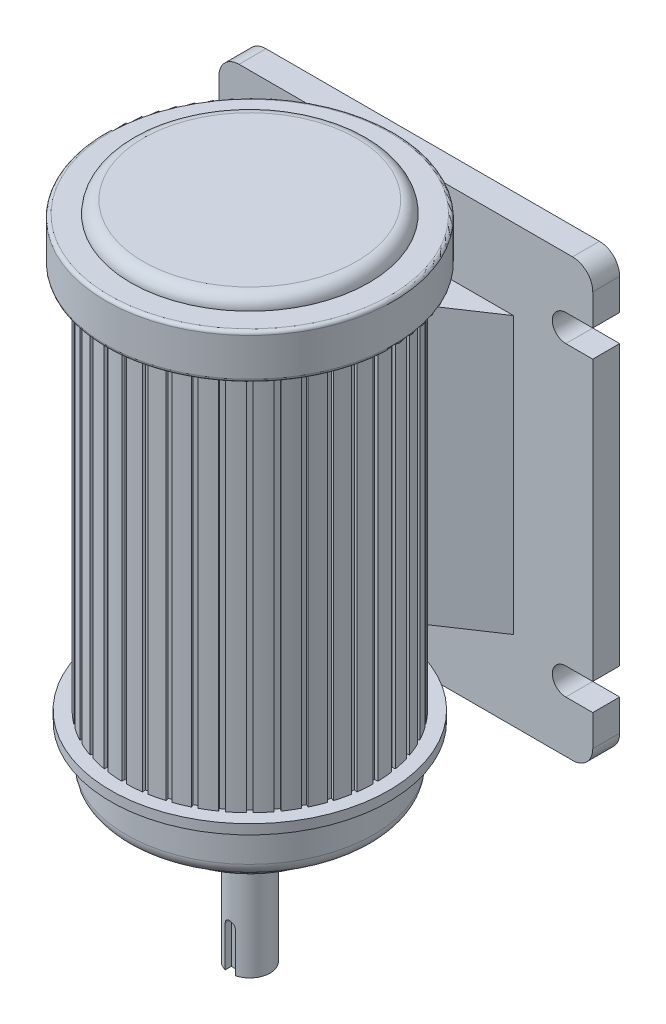
from build123d import *

# Parameters (mm, degrees)
SKETCH1_W           = 55.500789996
SKETCH1_H           = 64.737092018
BOSS_EXTRUDE1_DEPTH = 4
CUT_EXTRUDE1_DEPTH  = 4
FILLET1_R           = 3
CUT_EXTRUDE2_DEPTH  = 57.141911971
BOSS_EXTRUDE2_DEPTH = 20.5
SKETCH7_R           = 4.533623048
SKETCH7_R_2         = 3.951109074
BOSS_EXTRUDE3_DEPTH = 0.5
SKETCH8_R           = 3
BOSS_EXTRUDE4_DEPTH = 20
SKETCH9_W           = 1.5
SKETCH9_H           = 2
CUT_EXTRUDE3_DEPTH  = 6
SKETCH10_R          = 0.75
CUT_EXTRUDE4_DEPTH  = 2


with BuildPart() as part:
    # Sketch1 → Boss-Extrude1 (new body)
    with BuildSketch(Plane.XY):
        with Locations((9.22608239, 110.038628539)):
            Rectangle(SKETCH1_W, SKETCH1_H)
    extrude(amount=BOSS_EXTRUDE1_DEPTH)

    # Sketch2 → Cut-Extrude1 (cut)
    with BuildSketch(Plane.XY.offset(4)):
        with BuildLine():
            Line((-14.527141875, 134.7549071), (-18.524312608, 134.7549071))
            Line((-18.524312608, 134.7549071), (-18.524312608, 130.7549071))
            Line((-18.524312608, 130.7549071), (-14.527141875, 130.7549071))
            ThreePointArc((-14.527141875, 130.7549071), (-12.527141875, 132.7549071), (-14.527141875, 134.7549071))
        make_face()
        with BuildLine():
            Line((-18.524312608, 89.322349977), (-18.524312608, 85.322349977))
            Line((-18.524312608, 85.322349977), (-14.527141875, 85.322349977))
            ThreePointArc((-14.527141875, 85.322349977), (-12.527141875, 87.322349977), (-14.527141875, 89.322349977))
            Line((-14.527141875, 89.322349977), (-18.524312608, 89.322349977))
        make_face()
        with BuildLine():
            Line((36.976477388, 130.7549071), (36.976477388, 134.7549071))
            Line((36.976477388, 134.7549071), (32.979306656, 134.7549071))
            ThreePointArc((32.979306656, 134.7549071), (30.979306656, 132.7549071), (32.979306656, 130.7549071))
            Line((32.979306656, 130.7549071), (36.976477388, 130.7549071))
        make_face()
        with BuildLine():
            Line((36.976477388, 85.322349977), (36.976477388, 89.322349977))
            Line((36.976477388, 89.322349977), (32.979306656, 89.322349977))
            ThreePointArc((32.979306656, 89.322349977), (30.979306656, 87.322349977), (32.979306656, 85.322349977))
            Line((32.979306656, 85.322349977), (36.976477388, 85.322349977))
        make_face()
    extrude(amount=-CUT_EXTRUDE1_DEPTH, mode=Mode.SUBTRACT)

    # Fillet1
    fillet1_edges = [part.edges().sort_by_distance(p)[0] for p in [
        (36.976477388, 77.67008253, 2),
        (-18.524312608, 77.67008253, 2),
        (-18.524312608, 142.407174548, 2),
        (36.976477388, 142.407174548, 2),
    ]]
    fillet(fillet1_edges, radius=FILLET1_R)



with BuildPart() as body_2:
    # Sketch3 → Revolve1 (revolve)
    with BuildSketch(Plane(origin=(9.22608239, -4.248250363, 39.612036091), x_dir=(0, 1, 0), z_dir=(1, 0, 0)), mode=Mode.PRIVATE) as revolve1_sk:
        with BuildLine():
            Line((75.270637963, -12.45948374), (153.17887773, -12.45948374))
            Line((153.17887773, -12.45948374), (153.17887773, 3.386494149))
            ThreePointArc((153.17887773, 3.386494149), (152.644055983, 4.677668063), (151.352882069, 5.21248981))
            Line((151.352882069, 5.21248981), (151.352882069, 8.408578473))
            ThreePointArc((151.352882069, 8.408578473), (151.206435459, 8.762131864), (150.852882069, 8.908578473))
            Line((150.852882069, 8.908578473), (145.22638088, 8.908578473))
            ThreePointArc((145.22638088, 8.908578473), (144.872827489, 8.762131864), (144.72638088, 8.408578473))
            Line((144.72638088, 8.408578473), (144.72638088, 6.1906691))
            Line((144.72638088, 6.1906691), (87.584468909, 6.1906691))
            Line((87.584468909, 6.1906691), (87.584468909, 8.192651448))
            Line((87.584468909, 8.192651448), (86.141891274, 8.192651448))
            Line((86.141891274, 8.192651448), (86.141891274, 7.166046123))
            Line((86.141891274, 7.166046123), (86.141891274, 5.883061514))
            Line((86.141891274, 5.883061514), (80.722831843, 5.883061514))
            ThreePointArc((80.722831843, 5.883061514), (79.308618281, 5.297275076), (78.722831843, 3.883061514))
            Line((78.722831843, 3.883061514), (78.722831843, -0.040180747))
            Line((78.722831843, -0.040180747), (77.843708387, -0.682232562))
            Line((77.843708387, -0.682232562), (77.843708387, 0.737127384))
            ThreePointArc((77.843708387, 0.737127384), (77.785129743, 0.878548741), (77.643708387, 0.937127384))
            Line((77.643708387, 0.937127384), (76.752066951, 0.937127384))
            ThreePointArc((76.752066951, 0.937127384), (76.610645595, 0.878548741), (76.552066951, 0.737127384))
            Line((76.552066951, 0.737127384), (76.552066951, 0.029558387))
            Line((76.552066951, 0.029558387), (75.470637963, 0.029558387))
            ThreePointArc((75.470637963, 0.029558387), (75.329216607, -0.029020257), (75.270637963, -0.170441613))
            Line((75.270637963, -0.170441613), (75.270637963, -12.45948374))
        make_face()
    revolve(revolve1_sk.sketch.rotate(Axis((9.22608239, 71.0223876, 27.152552351), (0, 1, 0)), 180), axis=Axis((9.22608239, 71.0223876, 27.152552351), (0, 1, 0)))

    # Sketch5 → Cut-Extrude2 (cut)
    with BuildSketch(Plane(origin=(0, 83.336218546, 0), x_dir=(1, 0, 0), z_dir=(0, 1, 0))):
        with BuildLine():
            Line((11.788472717, -8.679264697), (11.714933059, -9.143575829))
            Line((11.714933059, -9.143575829), (12.424124541, -9.255900725))
            Line((12.424124541, -9.255900725), (12.4976642, -8.791589593))
            ThreePointArc((12.4976642, -8.791589593), (12.143609073, -8.732013841), (11.788472717, -8.679264697))
        make_face()
        with BuildLine():
            Line((8.867066569, -8.505855363), (8.867066569, -8.975954192))
            Line((8.867066569, -8.975954192), (9.585098212, -8.975954192))
            Line((9.585098212, -8.975954192), (9.585098212, -8.505855363))
            ThreePointArc((9.585098212, -8.505855363), (9.22608239, -8.502399512), (8.867066569, -8.505855363))
        make_face()
        with BuildLine():
            Line((14.646784312, -9.307547683), (14.501515785, -9.754638237))
            Line((14.501515785, -9.754638237), (15.184404458, -9.976522218))
            Line((15.184404458, -9.976522218), (15.329672985, -9.529431663))
            ThreePointArc((15.329672985, -9.529431663), (14.989296565, -9.415202963), (14.646784312, -9.307547683))
        make_face()
        with BuildLine():
            Line((17.371620235, -10.375233908), (17.158199833, -10.794095031))
            Line((17.158199833, -10.794095031), (17.797970712, -11.120074576))
            Line((17.797970712, -11.120074576), (18.011391114, -10.701213452))
            ThreePointArc((18.011391114, -10.701213452), (17.693074598, -10.535144494), (17.371620235, -10.375233908))
        make_face()
        with BuildLine():
            Line((19.895885983, -11.856033393), (19.619568824, -12.236351335))
            Line((19.619568824, -12.236351335), (20.200468626, -12.658399745))
            Line((20.200468626, -12.658399745), (20.476785785, -12.278081804))
            ThreePointArc((20.476785785, -12.278081804), (20.188367182, -12.064261756), (19.895885983, -11.856033393))
        make_face()
        with BuildLine():
            Line((22.157425755, -13.713483942), (21.825015686, -14.045894012))
            Line((21.825015686, -14.045894012), (22.33274073, -14.553619056))
            Line((22.33274073, -14.553619056), (22.6651508, -14.221208986))
            ThreePointArc((22.6651508, -14.221208986), (22.413731933, -13.964902808), (22.157425755, -13.713483942))
        make_face()
        with BuildLine():
            Line((24.100552937, -15.901848957), (23.720234996, -16.178166115))
            Line((23.720234996, -16.178166115), (24.142283407, -16.759065917))
            Line((24.142283407, -16.759065917), (24.522601348, -16.482748759))
            ThreePointArc((24.522601348, -16.482748759), (24.314372985, -16.190267559), (24.100552937, -15.901848957))
        make_face()
        with BuildLine():
            Line((25.677421289, -18.367243628), (25.258560166, -18.58066403))
            Line((25.258560166, -18.58066403), (25.58453971, -19.220434909))
            Line((25.58453971, -19.220434909), (26.003400834, -19.007014506))
            ThreePointArc((26.003400834, -19.007014506), (25.843490247, -18.685560143), (25.677421289, -18.367243628))
        make_face()
        with BuildLine():
            Line((26.849203078, -21.048961756), (26.402112524, -21.194230283))
            Line((26.402112524, -21.194230283), (26.623996504, -21.877118957))
            Line((26.623996504, -21.877118957), (27.071087059, -21.73185043))
            ThreePointArc((27.071087059, -21.73185043), (26.963431778, -21.389338176), (26.849203078, -21.048961756))
        make_face()
        with BuildLine():
            Line((27.587045148, -23.880970542), (27.122734016, -23.954510201))
            Line((27.122734016, -23.954510201), (27.235058912, -24.663701683))
            Line((27.235058912, -24.663701683), (27.699370044, -24.590162024))
            ThreePointArc((27.699370044, -24.590162024), (27.6466209, -24.235025669), (27.587045148, -23.880970542))
        make_face()
        with BuildLine():
            Line((27.872779379, -26.79353653), (27.40268055, -26.79353653))
            Line((27.40268055, -26.79353653), (27.40268055, -27.511568173))
            Line((27.40268055, -27.511568173), (27.872779379, -27.511568173))
            ThreePointArc((27.872779379, -27.511568173), (27.87623523, -27.152552351), (27.872779379, -26.79353653))
        make_face()
        with BuildLine():
            Line((27.699370044, -29.714942678), (27.235058912, -29.641403019))
            Line((27.235058912, -29.641403019), (27.122734016, -30.350594502))
            Line((27.122734016, -30.350594502), (27.587045148, -30.42413416))
            ThreePointArc((27.587045148, -30.42413416), (27.6466209, -30.070079034), (27.699370044, -29.714942678))
        make_face()
        with BuildLine():
            Line((27.071087059, -32.573254273), (26.623996504, -32.427985746))
            Line((26.623996504, -32.427985746), (26.402112524, -33.110874419))
            Line((26.402112524, -33.110874419), (26.849203078, -33.256142946))
            ThreePointArc((26.849203078, -33.256142946), (26.963431778, -32.915766526), (27.071087059, -32.573254273))
        make_face()
        with BuildLine():
            Line((26.003400834, -35.298090196), (25.58453971, -35.084669794))
            Line((25.58453971, -35.084669794), (25.258560166, -35.724440673))
            Line((25.258560166, -35.724440673), (25.677421289, -35.937861075))
            ThreePointArc((25.677421289, -35.937861075), (25.843490247, -35.619544559), (26.003400834, -35.298090196))
        make_face()
        with BuildLine():
            Line((24.522601348, -37.822355944), (24.142283407, -37.546038785))
            Line((24.142283407, -37.546038785), (23.720234996, -38.126938587))
            Line((23.720234996, -38.126938587), (24.100552937, -38.403255746))
            ThreePointArc((24.100552937, -38.403255746), (24.314372985, -38.114837143), (24.522601348, -37.822355944))
        make_face()
        with BuildLine():
            Line((22.6651508, -40.083895716), (22.33274073, -39.751485647))
            Line((22.33274073, -39.751485647), (21.825015686, -40.259210691))
            Line((21.825015686, -40.259210691), (22.157425755, -40.59162076))
            ThreePointArc((22.157425755, -40.59162076), (22.413731933, -40.340201894), (22.6651508, -40.083895716))
        make_face()
        with BuildLine():
            Line((20.476785785, -42.027022898), (20.200468626, -41.646704957))
            Line((20.200468626, -41.646704957), (19.619568824, -42.068753368))
            Line((19.619568824, -42.068753368), (19.895885983, -42.449071309))
            ThreePointArc((19.895885983, -42.449071309), (20.188367182, -42.240842946), (20.476785785, -42.027022898))
        make_face()
        with BuildLine():
            Line((18.011391114, -43.60389125), (17.797970712, -43.185030127))
            Line((17.797970712, -43.185030127), (17.158199833, -43.511009671))
            Line((17.158199833, -43.511009671), (17.371620235, -43.929870795))
            ThreePointArc((17.371620235, -43.929870795), (17.693074598, -43.769960208), (18.011391114, -43.60389125))
        make_face()
        with BuildLine():
            Line((15.329672985, -44.775673039), (15.184404458, -44.328582485))
            Line((15.184404458, -44.328582485), (14.501515785, -44.550466465))
            Line((14.501515785, -44.550466465), (14.646784312, -44.997557019))
            ThreePointArc((14.646784312, -44.997557019), (14.989296565, -44.889901739), (15.329672985, -44.775673039))
        make_face()
        with BuildLine():
            Line((12.4976642, -45.513515109), (12.424124541, -45.049203977))
            Line((12.424124541, -45.049203977), (11.714933059, -45.161528873))
            Line((11.714933059, -45.161528873), (11.788472717, -45.625840005))
            ThreePointArc((11.788472717, -45.625840005), (12.143609073, -45.573090861), (12.4976642, -45.513515109))
        make_face()
        with BuildLine():
            Line((9.585098212, -45.799249339), (9.585098212, -45.329150511))
            Line((9.585098212, -45.329150511), (8.867066569, -45.329150511))
            Line((8.867066569, -45.329150511), (8.867066569, -45.799249339))
            ThreePointArc((8.867066569, -45.799249339), (9.22608239, -45.802705191), (9.585098212, -45.799249339))
        make_face()
        with BuildLine():
            Line((6.663692063, -45.625840005), (6.737231722, -45.161528873))
            Line((6.737231722, -45.161528873), (6.02804024, -45.049203977))
            Line((6.02804024, -45.049203977), (5.954500581, -45.513515109))
            ThreePointArc((5.954500581, -45.513515109), (6.308555708, -45.573090861), (6.663692063, -45.625840005))
        make_face()
        with BuildLine():
            Line((3.805380469, -44.997557019), (3.950648996, -44.550466465))
            Line((3.950648996, -44.550466465), (3.267760322, -44.328582485))
            Line((3.267760322, -44.328582485), (3.122491795, -44.775673039))
            ThreePointArc((3.122491795, -44.775673039), (3.462868215, -44.889901739), (3.805380469, -44.997557019))
        make_face()
        with BuildLine():
            Line((1.080544546, -43.929870795), (1.293964948, -43.511009671))
            Line((1.293964948, -43.511009671), (0.654194069, -43.185030127))
            Line((0.654194069, -43.185030127), (0.440773667, -43.60389125))
            ThreePointArc((0.440773667, -43.60389125), (0.759090183, -43.769960208), (1.080544546, -43.929870795))
        make_face()
        with BuildLine():
            Line((-1.443721202, -42.449071309), (-1.167404044, -42.068753368))
            Line((-1.167404044, -42.068753368), (-1.748303846, -41.646704957))
            Line((-1.748303846, -41.646704957), (-2.024621004, -42.027022898))
            ThreePointArc((-2.024621004, -42.027022898), (-1.736202402, -42.240842946), (-1.443721202, -42.449071309))
        make_face()
        with BuildLine():
            Line((-3.705260975, -40.59162076), (-3.372850905, -40.259210691))
            Line((-3.372850905, -40.259210691), (-3.880575949, -39.751485647))
            Line((-3.880575949, -39.751485647), (-4.212986019, -40.083895716))
            ThreePointArc((-4.212986019, -40.083895716), (-3.961567152, -40.340201894), (-3.705260975, -40.59162076))
        make_face()
        with BuildLine():
            Line((-5.648388157, -38.403255746), (-5.268070215, -38.126938587))
            Line((-5.268070215, -38.126938587), (-5.690118626, -37.546038785))
            Line((-5.690118626, -37.546038785), (-6.070436567, -37.822355944))
            ThreePointArc((-6.070436567, -37.822355944), (-5.862208204, -38.114837143), (-5.648388157, -38.403255746))
        make_face()
        with BuildLine():
            Line((-7.225256508, -35.937861075), (-6.806395385, -35.724440673))
            Line((-6.806395385, -35.724440673), (-7.13237493, -35.084669794))
            Line((-7.13237493, -35.084669794), (-7.551236053, -35.298090196))
            ThreePointArc((-7.551236053, -35.298090196), (-7.391325467, -35.619544559), (-7.225256508, -35.937861075))
        make_face()
        with BuildLine():
            Line((-8.397038297, -33.256142946), (-7.949947743, -33.110874419))
            Line((-7.949947743, -33.110874419), (-8.171831724, -32.427985746))
            Line((-8.171831724, -32.427985746), (-8.618922278, -32.573254273))
            ThreePointArc((-8.618922278, -32.573254273), (-8.511266997, -32.915766526), (-8.397038297, -33.256142946))
        make_face()
        with BuildLine():
            Line((-9.134880367, -30.42413416), (-8.670569236, -30.350594502))
            Line((-8.670569236, -30.350594502), (-8.782894132, -29.641403019))
            Line((-8.782894132, -29.641403019), (-9.247205263, -29.714942678))
            ThreePointArc((-9.247205263, -29.714942678), (-9.194456119, -30.070079034), (-9.134880367, -30.42413416))
        make_face()
        with BuildLine():
            Line((-9.420614598, -27.511568173), (-8.950515769, -27.511568173))
            Line((-8.950515769, -27.511568173), (-8.950515769, -26.79353653))
            Line((-8.950515769, -26.79353653), (-9.420614598, -26.79353653))
            ThreePointArc((-9.420614598, -26.79353653), (-9.424070449, -27.152552351), (-9.420614598, -27.511568173))
        make_face()
        with BuildLine():
            Line((-9.247205263, -24.590162024), (-8.782894132, -24.663701683))
            Line((-8.782894132, -24.663701683), (-8.670569236, -23.954510201))
            Line((-8.670569236, -23.954510201), (-9.134880367, -23.880970542))
            ThreePointArc((-9.134880367, -23.880970542), (-9.194456119, -24.235025669), (-9.247205263, -24.590162024))
        make_face()
        with BuildLine():
            Line((-8.618922278, -21.73185043), (-8.171831724, -21.877118957))
            Line((-8.171831724, -21.877118957), (-7.949947743, -21.194230283))
            Line((-7.949947743, -21.194230283), (-8.397038297, -21.048961756))
            ThreePointArc((-8.397038297, -21.048961756), (-8.511266997, -21.389338176), (-8.618922278, -21.73185043))
        make_face()
        with BuildLine():
            Line((-7.551236053, -19.007014506), (-7.13237493, -19.220434909))
            Line((-7.13237493, -19.220434909), (-6.806395385, -18.58066403))
            Line((-6.806395385, -18.58066403), (-7.225256508, -18.367243628))
            ThreePointArc((-7.225256508, -18.367243628), (-7.391325467, -18.685560143), (-7.551236053, -19.007014506))
        make_face()
        with BuildLine():
            Line((-6.070436567, -16.482748759), (-5.690118626, -16.759065917))
            Line((-5.690118626, -16.759065917), (-5.268070215, -16.178166115))
            Line((-5.268070215, -16.178166115), (-5.648388157, -15.901848957))
            ThreePointArc((-5.648388157, -15.901848957), (-5.862208204, -16.190267559), (-6.070436567, -16.482748759))
        make_face()
        with BuildLine():
            Line((-4.212986019, -14.221208986), (-3.880575949, -14.553619056))
            Line((-3.880575949, -14.553619056), (-3.372850905, -14.045894012))
            Line((-3.372850905, -14.045894012), (-3.705260975, -13.713483942))
            ThreePointArc((-3.705260975, -13.713483942), (-3.961567152, -13.964902808), (-4.212986019, -14.221208986))
        make_face()
        with BuildLine():
            Line((-2.024621004, -12.278081804), (-1.748303846, -12.658399745))
            Line((-1.748303846, -12.658399745), (-1.167404044, -12.236351335))
            Line((-1.167404044, -12.236351335), (-1.443721202, -11.856033393))
            ThreePointArc((-1.443721202, -11.856033393), (-1.736202402, -12.064261756), (-2.024621004, -12.278081804))
        make_face()
        with BuildLine():
            Line((0.440773667, -10.701213452), (0.654194069, -11.120074576))
            Line((0.654194069, -11.120074576), (1.293964948, -10.794095031))
            Line((1.293964948, -10.794095031), (1.080544546, -10.375233908))
            ThreePointArc((1.080544546, -10.375233908), (0.759090183, -10.535144494), (0.440773667, -10.701213452))
        make_face()
        with BuildLine():
            Line((3.122491795, -9.529431663), (3.267760322, -9.976522218))
            Line((3.267760322, -9.976522218), (3.950648996, -9.754638237))
            Line((3.950648996, -9.754638237), (3.805380469, -9.307547683))
            ThreePointArc((3.805380469, -9.307547683), (3.462868215, -9.415202963), (3.122491795, -9.529431663))
        make_face()
        with BuildLine():
            Line((5.954500581, -8.791589593), (6.02804024, -9.255900725))
            Line((6.02804024, -9.255900725), (6.737231722, -9.143575829))
            Line((6.737231722, -9.143575829), (6.663692063, -8.679264697))
            ThreePointArc((6.663692063, -8.679264697), (6.308555708, -8.732013841), (5.954500581, -8.791589593))
        make_face()
    extrude(amount=CUT_EXTRUDE2_DEPTH, mode=Mode.SUBTRACT)


with BuildPart() as part_1:
    add(part.part)

    add(body_2.part)  # Boss-Extrude2 merges body 2
    # Sketch6 → Boss-Extrude2 (add, symmetric)
    with BuildSketch(Plane(origin=(0, 109.976507483, 0), x_dir=(1, 0, 0), z_dir=(0, 1, 0))):
        Polygon((-6.770913855, -4), (9.22608239, -14.710941589), (25.223078635, -4), align=None)
    extrude(amount=BOSS_EXTRUDE2_DEPTH, both=True)

    # Sketch7 → Boss-Extrude3 (add, symmetric)
    with BuildSketch(Plane.XZ.offset(-71.0223876)):
        with Locations(Location((9.22608239, 27.152552351, 0), (0, 0, 90))):
            Circle(SKETCH7_R)
        with Locations(Location((9.22608239, 27.152552351, 0), (0, 0, 90))):
            Circle(SKETCH7_R_2, mode=Mode.SUBTRACT)
    extrude(amount=BOSS_EXTRUDE3_DEPTH, both=True)

    # Sketch8 → Boss-Extrude4 (add)
    with BuildSketch(Plane.XZ.offset(-71.0223876)):
        with Locations(Location((9.22608239, 27.152552351, 0), (0, 0, 90))):
            Circle(SKETCH8_R)
    extrude(amount=BOSS_EXTRUDE4_DEPTH)

    # Sketch9 → Cut-Extrude3 (cut)
    with BuildSketch(Plane.XZ.offset(-51.0223876)):
        with Locations((9.22608239, 30.152552351)):
            Rectangle(SKETCH9_W, SKETCH9_H)
    extrude(amount=-CUT_EXTRUDE3_DEPTH, mode=Mode.SUBTRACT)

    # Sketch10 → Cut-Extrude4 (cut)
    with BuildSketch(Plane.XY.offset(29.152552351)):
        with Locations((9.22608239, 57.0223876)):
            Circle(SKETCH10_R)
    extrude(amount=CUT_EXTRUDE4_DEPTH, mode=Mode.SUBTRACT)


solid = part_1.part
